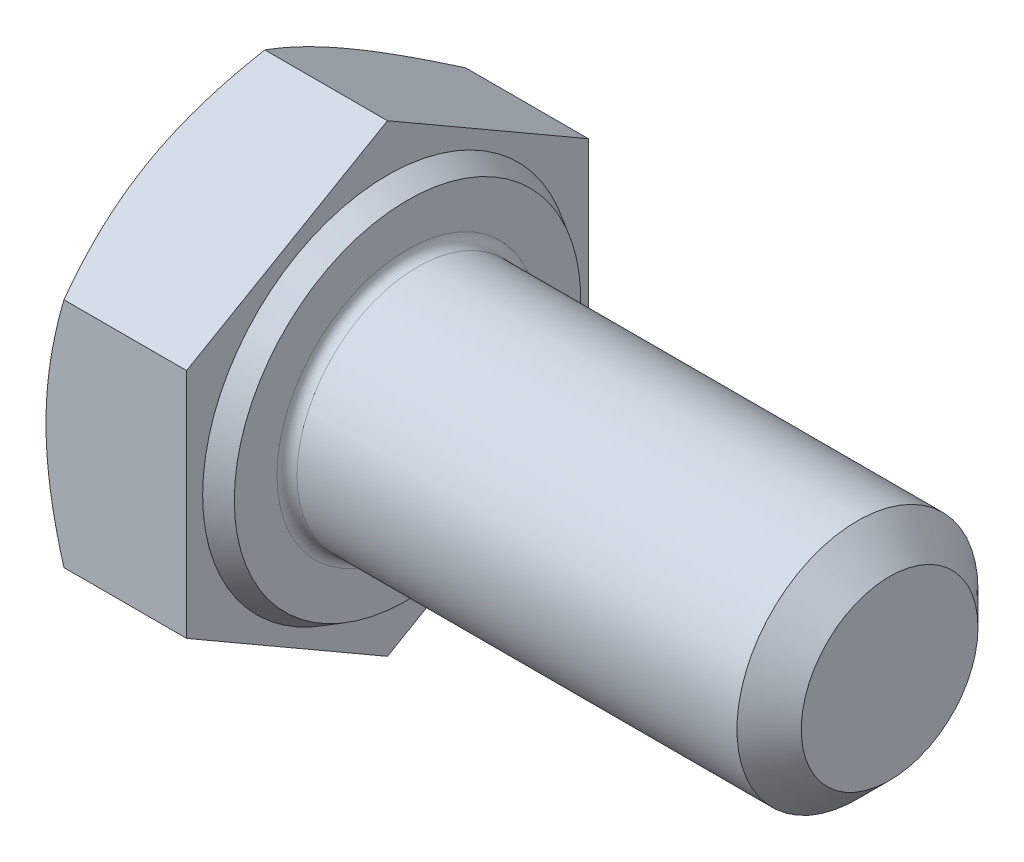
SolidWorks part; units mm, degrees
ref_plane "Front Plane" through (0, 0, 0) normal (0, 0, 1) x (1, 0, 0)
ref_plane "Top Plane" through (0, 0, 0) normal (0, 1, 0) x (1, 0, 0)
ref_plane "Right Plane" through (0, 0, 0) normal (1, 0, 0) x (0, 0, -1)
sketch "Dimension sketch" plane through (0, 0, 0) normal (0, 0, 1) x (1, 0, 0)
  line L0 (0, 0) -> (12, 0) construction
  line L1 (0, 0) -> (0, 6) construction
  point P3 (1, 0)
  point P4 (0.5, 0)
  point P6 (0, 7.2)
  point P7 (0, 6.48)
  point P8 (0, 8.74)
  point P9 (10.89, 0)
  point P10 (4, 0)
  point P11 (2.54, 0)
  point P12 (0.25, 0)
  point P13 (10, 0)
  point P14 (12, 0)
  point P15 (9, 0)
  point P16 (21, 0)
  dimension "b(参考)" = 12
  dimension "P" = 1
  dimension "d" = 6
  dimension "c(max)" = 0.5
  dimension "da(max)" = 7.2
  dimension "ds(max)" = 6.48
  dimension "dw(min)" = 8.74
  dimension "e(min)" = 10.89
  dimension "k(公称)" = 4
  dimension "kw(min)" = 2.54
  dimension "r(min)" = 0.25
  dimension "s(公称)" = 10
  dimension "l" = 12
sketch "Sketch1" plane through (0, 0, 0) normal (1, 0, 0) x (0, 0, -1)
  line L0 (5, 2.8868) -> (5, -2.8868)
  line L1 (-5, 2.8868) -> (-5, -2.8868)
  line L2 (5, -2.8868) -> (0, -5.7735)
  line L3 (0, -5.7735) -> (-5, -2.8868)
  line L4 (5, 2.8868) -> (0, 5.7735)
  line L5 (0, 5.7735) -> (-5, 2.8868)
  point P6 (0, 5.1165)
  dimension "D1" = 10.89
  dimension "s" = 10
  dimension "D2" = 120
  dimension "D3" = 5
  dimension "D4" = 5
  dimension "D5" = 5
extrude "Base-extrude" add sketch "Sketch1" along normal blind 4
sketch "Sketch2" plane through (0, 0, 0) normal (0, 0, 1) x (1, 0, 0)
  line L0 (0, 2.8868) -> (0, -2.8868) construction
  line L1 (0, 0) -> (16, 0)
  line L2 (0, 0) -> (0, 3)
  line L3 (0, 3) -> (4, 3)
  line L4 (16, 0) -> (16, 2.134)
  line L5 (4, 5.7735) -> (4, 2.8868) construction
  line L7 (0, 0) -> (-51.1435, 0) construction
  line L8 (16, -2.134) -> (4, -3) construction
  line L9 (0, -3) -> (4, -3) construction
  line L10 (5, 3) -> (5, 0) construction
  line L11 (4, 3) -> (4, 0) construction
  line L12 (4, 2.8868) -> (4, -2.8868) construction
  line L13 (4, 3) -> (16, 3)
  line L14 (16, 3) -> (16, 2.134)
  dimension "l" = 12
  dimension "d" = 6
  dimension "Minor_dia" = 4.268
  dimension "p" = 1
  dimension "b" = 12
revolve "Boss-Revolve1" add sketch "Sketch2" angle 360 about L7
cosmetic thread "Cosmetic Thread1" parameters "D1"=11.45, "D2"=4.8
sketch "Sketch3" plane through (0, 0, 0) normal (0, 0, 1) x (1, 0, 0)
  line L0 (0, 5) -> (3.3333, 10.7735)
  line L1 (0, 5.7735) -> (0, 2.8868) construction
  line L2 (3.3333, 10.7735) -> (3.3333, 15.7735)
  line L3 (3.3333, 15.7735) -> (-10, 15.7735)
  line L4 (-10, 15.7735) -> (-10, 5)
  line L5 (-10, 5) -> (0, 5)
  line L6 (0, 0) -> (99.06, 0) construction
  line L7 (4, 5.7735) -> (0, 5.7735) construction
  dimension "D1" = 5
  dimension "D2" = 5
  dimension "D3" = 10
  dimension "D4" = 5
  dimension "Head_ch_ang" = 30
revolve "Cut-Revolve1" cut sketch "Sketch3" angle 360 about L6
sketch "Sketch5" plane through (0, 0, 0) normal (0, 0, 1) x (1, 0, 0)
  line L0 (4, 5) -> (0.6667, 10.7735)
  line L1 (4, 5.7735) -> (4, 2.8868) construction
  line L2 (0.6667, 10.7735) -> (0.6667, 15.7735)
  line L3 (0.6667, 15.7735) -> (10.6667, 15.7735)
  line L4 (10.6667, 15.7735) -> (10.6667, 5)
  line L5 (10.6667, 5) -> (4, 5)
  line L7 (4, 5.7735) -> (0.4466, 5.7735) construction
  line L8 (0, 0) -> (99.06, 0) construction
  line L9 (0, 0) -> (99.06, 0) construction
  dimension "D1" = 5
  dimension "D2" = 5
  dimension "D3" = 10
  dimension "Head_ch_ang" = 30
  dimension "D4" = 5
revolve "Cut-Revolve2" cut sketch "Sketch5" angle 360 about L8
sketch "Sketch4" plane through (0, 0, 0) normal (0, 0, 1) x (1, 0, 0)
  line L0 (3.9, 4.37) -> (3.9, 0) construction
  line L1 (4, 5.7735) -> (4, 2.8868) construction
  line L2 (4, 4.3123) -> (3.5, 4.6009)
  line L3 (4, 4.3123) -> (4, 15.7735)
  line L4 (4, 15.7735) -> (3.5, 15.7735)
  line L5 (0, 0) -> (95.25, 0) construction
  line L6 (-51.1435, 0) -> (0, 0) construction
  line L7 (3.5, 4.6009) -> (3.5, 15.7735)
  line L8 (3.5534, 5.7735) -> (0.4466, 5.7735) construction
  line L9 (4, 4.3301) -> (4, 5) construction
  line L10 (3.5534, 5.7735) -> (0.4466, 5.7735) construction
  point P15 (1.36, 5.7735)
  dimension "D1" = 120
  dimension "D2" = 10
  dimension "D3" = 0.1
  dimension "c" = 0.5
  dimension "D4" = 8.74
  dimension "D5" = 2.54
revolve "Cut-Revolve3" cut sketch "Sketch4" angle 360 about L5
chamfer "Chamfer" distance 0.8 angle 45 1 edges at (16, 0, -3)
sketch "Sketch9" plane through (0, 0, 0) normal (0, 0, 1) x (1, 0, 0)
  line L0 (4, -4.3123) -> (4, 4.3123) construction
  line L1 (15.2, 3) -> (4, 3) construction
  line L2 (0, 0) -> (4, 0) construction
  line L3 (4, 3.25) -> (4, 3)
  line L4 (4, 3) -> (4.25, 3)
  arc A0 (4, 3.25) -> (4.25, 3) centre (4.25, 3.25) ccw
  dimension "D1" = 0.25
revolve "Revolve1" add sketch "Sketch9" angle 360 about L2
sketch "Sketch6" plane through (0, 0, 0) normal (0, 0, 1) x (1, 0, 0)
  line L0 (14.7, -2.134) -> (14.2, -3)
  line L1 (14.7, -2.134) -> (15.2, -3)
  line L2 (15.2, -3) -> (15.2, -5.7735)
  line L3 (-3.175, 0) -> (0, 0) construction
  line L4 (15.2, -3) -> (15.2, 3) construction
  line L5 (15.2, -5.7735) -> (14.2, -5.7735)
  line L6 (14.2, -5.7735) -> (14.2, -3)
  line L7 (4.25, -3) -> (15.2, -3) construction
  line L9 (3.5, -5.7735) -> (0.4466, -5.7735) construction
  dimension "Thread_minor" = 4.268
  dimension "SideAngle" = 60
  dimension "VeeAngle" = 60
